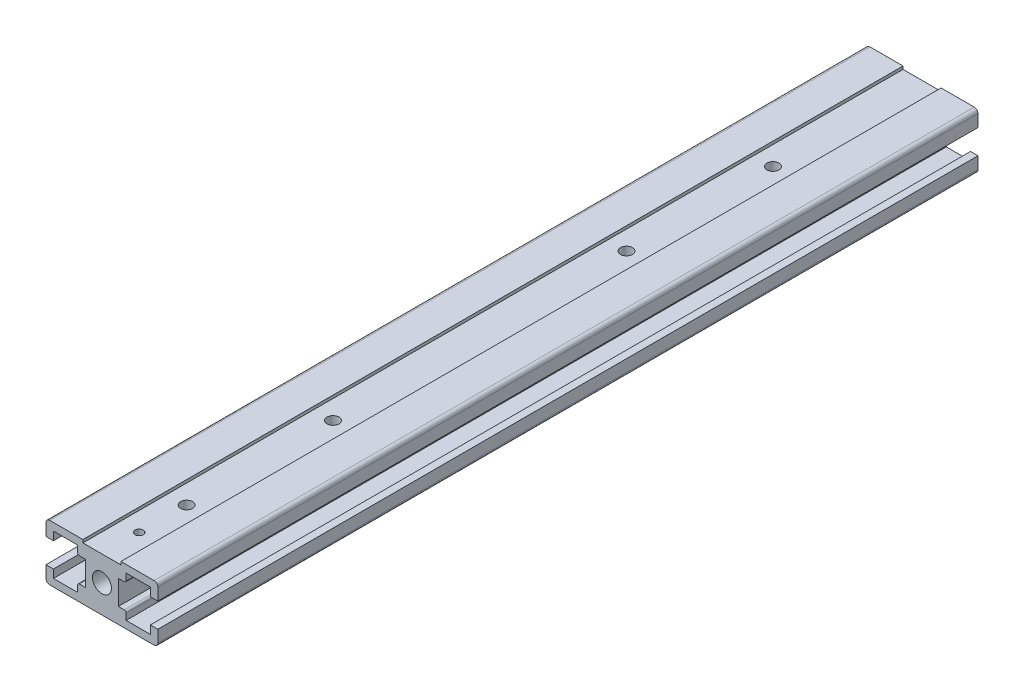
SolidWorks part; units mm, degrees
ref_plane "前视基准面" through (0, 0, 0) normal (0, 0, 1) x (1, 0, 0)
ref_plane "上视基准面" through (0, 0, 0) normal (0, 1, 0) x (1, 0, 0)
ref_plane "右视基准面" through (0, 0, 0) normal (1, 0, 0) x (0, 0, -1)
sketch "草图1" plane through (0, 0, 0) normal (0, 0, 1) x (1, 0, 0)
  line L1 (-15, 7.5) -> (15, 7.5)
  line L2 (-15, 7.5) -> (-15, -7.5)
  line L3 (-15, -7.5) -> (15, -7.5)
  line L4 (15, 7.5) -> (15, -7.5)
  line L5 (-15, 7.5) -> (15, -7.5) construction
  line L6 (-15, -7.5) -> (15, 7.5) construction
  point P0 (0, 0)
  dimension "D1" = 30
  dimension "D2" = 15
extrude "凸台-拉伸1" add sketch "草图1" along normal blind 220
fillet "圆角1" radius 1 4 edges at (15, -7.5, 110) (-15, -7.5, 110) (-15, 7.5, 110) (15, 7.5, 110)
sketch "草图2" plane through (0, 0, 220) normal (0, 0, 1) x (1, 0, 0)
  circle A0 centre (0, 0) radius 2.55
extrude "切除-拉伸1" cut sketch "草图2" against normal blind 230
sketch "草图3" plane through (0, 0, 220) normal (0, 0, 1) x (1, 0, 0)
  line L0 (-15, 6.5) -> (-15, -6.5) construction
  line L1 (-25.6, 3.25) -> (-4.4, 3.25)
  line L2 (-25.6, 3.25) -> (-25.6, -3.3)
  line L3 (-25.6, -3.3) -> (-4.4, -3.3)
  line L4 (-4.4, 3.25) -> (-4.4, -3.3)
  line L5 (-25.6, 3.25) -> (-4.4, -3.3) construction
  line L6 (-25.6, -3.3) -> (-4.4, 3.25) construction
  line L7 (14, 7.5) -> (-14, 7.5) construction
  point P0 (-15, 0)
  dimension "D1" = 6.55
  dimension "D2" = 10.6
  dimension "D3" = 4.25
extrude "切除-拉伸2" cut sketch "草图3" against normal blind 230
mirror "镜向1" about plane through (0, 0, 0) normal (1, 0, 0) of "切除-拉伸2"
sketch "草图4" plane through (0, 0, 220) normal (0, 0, 1) x (1, 0, 0)
  line L0 (-15, 6.5) -> (-15, 3.25) construction
  line L1 (-13, 5.5) -> (-6.5, 5.5)
  line L2 (-13, 5.5) -> (-13, -5.5)
  line L3 (-13, -5.5) -> (-6.5, -5.5)
  line L4 (-6.5, 5.5) -> (-6.5, -5.5)
  line L5 (14, 7.5) -> (-14, 7.5) construction
  line L6 (-14, -7.5) -> (14, -7.5) construction
  dimension "D1" = 2
  dimension "D2" = 2
  dimension "D3" = 6.5
  dimension "D4" = 2
extrude "切除-拉伸3" cut sketch "草图4" against normal blind 230
mirror "镜向2" about plane through (0, 0, 0) normal (1, 0, 0) of "切除-拉伸3"
fillet "圆角2" radius 0.5 4 edges at (-6.5, -3.3, 110) (-6.5, 3.25, 110) (6.5, -3.3, 110) (6.5, 3.25, 110)
sketch "草图5" plane through (0, 7.5, 0) normal (0, 1, 0) x (1, 0, 0)
  line L1 (14, 0) -> (-14, 0) construction
  circle A0 centre (0, -40) radius 1.6
  circle A1 centre (0, -79.2857) radius 1.6
  dimension "D1" = 3.2
  dimension "D2" = 3.2
  dimension "D4" = 40
  dimension "D3" = 39.2857
extrude "切除-拉伸4" cut sketch "草图5" against normal blind 10
pattern_linear "阵列(线性)1" count 2 spacing 118 along (0, 0, 1) of "切除-拉伸4"
sketch "草图6" plane through (0, 7.5, 0) normal (0, 1, 0) x (1, 0, 0)
  line L0 (14, -220) -> (-14, -220) construction
  circle A0 centre (0, -210) radius 1.1
  dimension "D2" = 2.2
  dimension "D1" = 10
extrude "切除-拉伸5" cut sketch "草图6" against normal through all
sketch "草图7" plane through (0, 7.5, 0) normal (0, 1, 0) x (1, 0, 0)
  line L0 (14, 0) -> (-14, 0) construction
  line L1 (-5.1, 0) -> (5.1, 0)
  line L2 (-5.1, 0) -> (-5.1, -220)
  line L3 (-5.1, -220) -> (5.1, -220)
  line L4 (5.1, 0) -> (5.1, -220)
  line L5 (14, -220) -> (-14, -220) construction
  circle A0 centre (0, -210) radius 1.1 construction
  dimension "D1" = 10.2
  dimension "D2" = 5.1
extrude "切除-拉伸6" cut sketch "草图7" against normal blind 0.8
